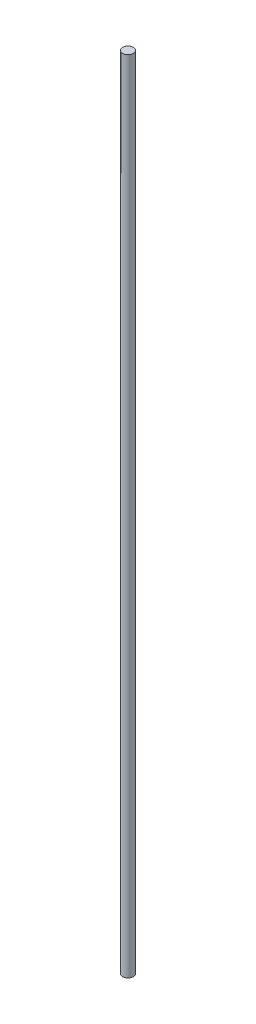
SolidWorks part; units mm, degrees
ref_plane "Front Plane" through (0, 0, 0) normal (0, 0, 1) x (1, 0, 0)
ref_plane "Top Plane" through (0, 0, 0) normal (0, 1, 0) x (1, 0, 0)
ref_plane "Right Plane" through (0, 0, 0) normal (1, 0, 0) x (0, 0, -1)
sketch "Sketch1" plane through (0, 0, 0) normal (0, 1, 0) x (1, 0, 0)
  circle A0 centre (0, 0) radius 4
  dimension "D1" = 8
extrude "Boss-Extrude1" add sketch "Sketch1" along normal blind 600
